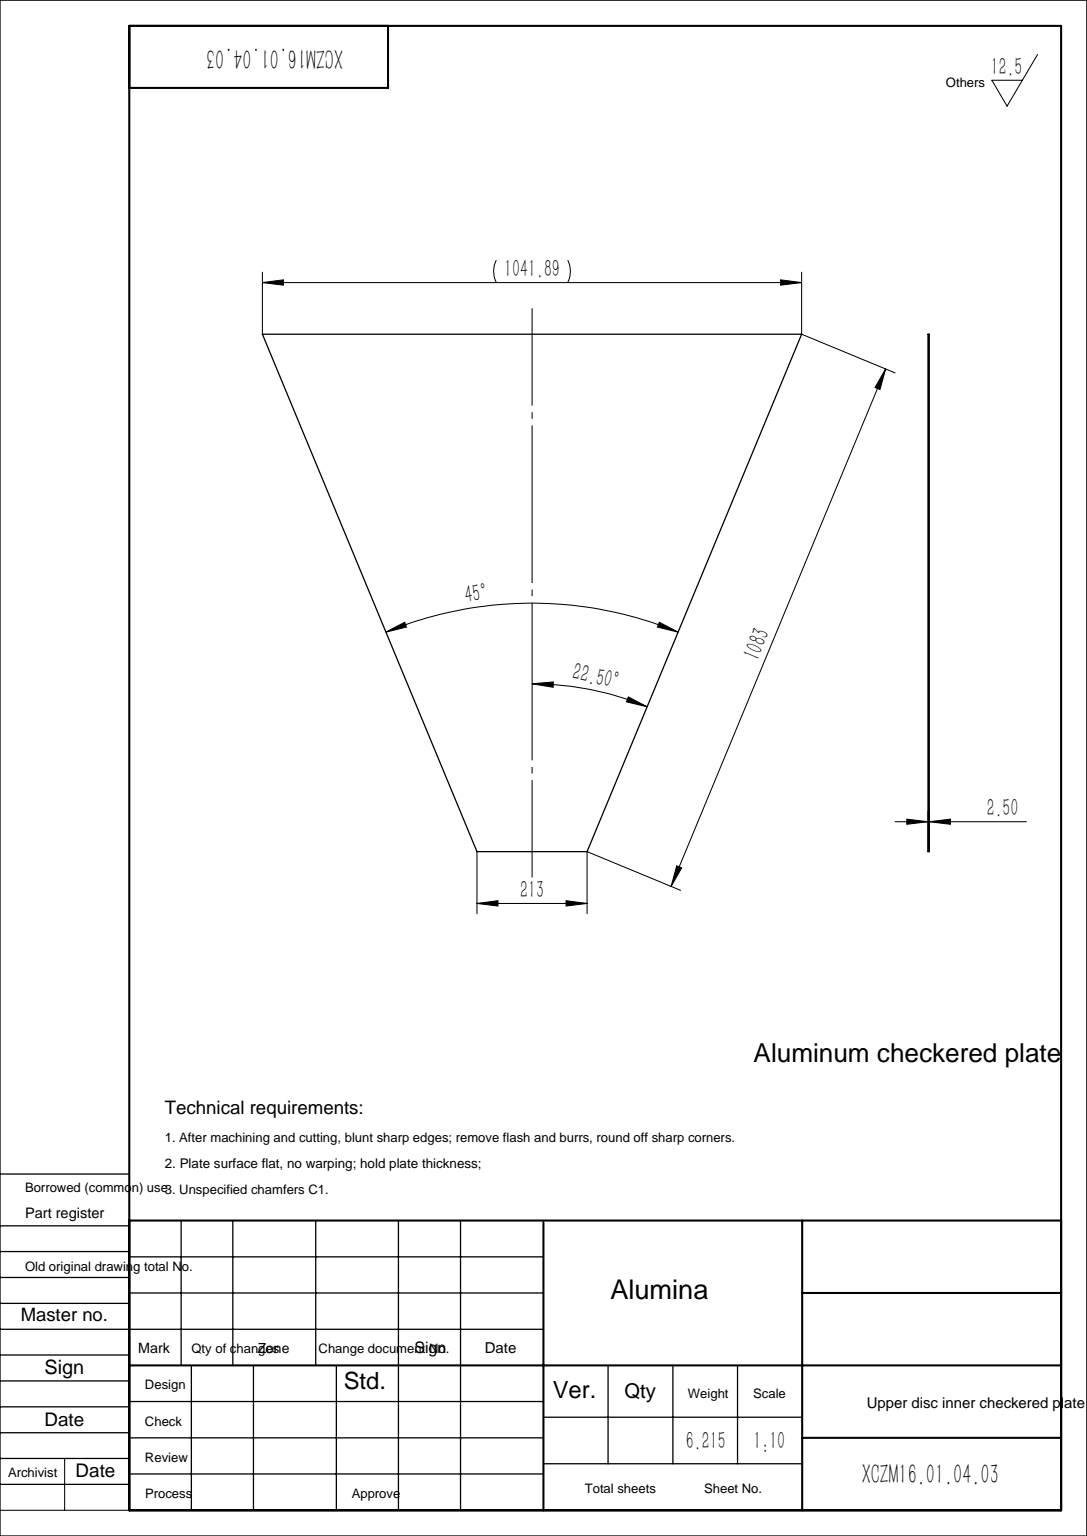
SolidWorks part; units mm, degrees
material "Alumina"
ref_plane "Front Plane" through (0, 0, 0) normal (0, 0, 1) x (1, 0, 0)
ref_plane "Top Plane" through (0, 0, 0) normal (0, 1, 0) x (1, 0, 0)
ref_plane "Right Plane" through (0, 0, 0) normal (1, 0, 0) x (0, 0, -1)
sketch "Sketch1" plane through (0, 0, 0) normal (0, 0, 1) x (1, 0, 0)
  line L0 (0, 0) -> (0, 1104.1842) construction
  line L1 (-106.5, 0) -> (106.5, 0)
  line L2 (106.5, 0) -> (520.9462, 1000.5615)
  line L3 (-106.5, 0) -> (-520.9462, 1000.5615)
  line L4 (-520.9462, 1000.5615) -> (520.9462, 1000.5615)
  arc A0 (520.9462, 1000.5615) -> (0, 1104.1842) centre (0, -257.1137) ccw
  arc A1 (-520.9462, 1000.5615) -> (0, 1104.1842) centre (0, -257.1137) cw
  dimension "D1" = 213
  dimension "D2" = 45
  dimension "D3" = 1083
  dimension "D4" = 1041.8923
extrude "Boss-Extrude1" add sketch "Sketch1" along normal blind 2.5 contours L0 L1 L2 L4 | L1 L0 L4 L3
